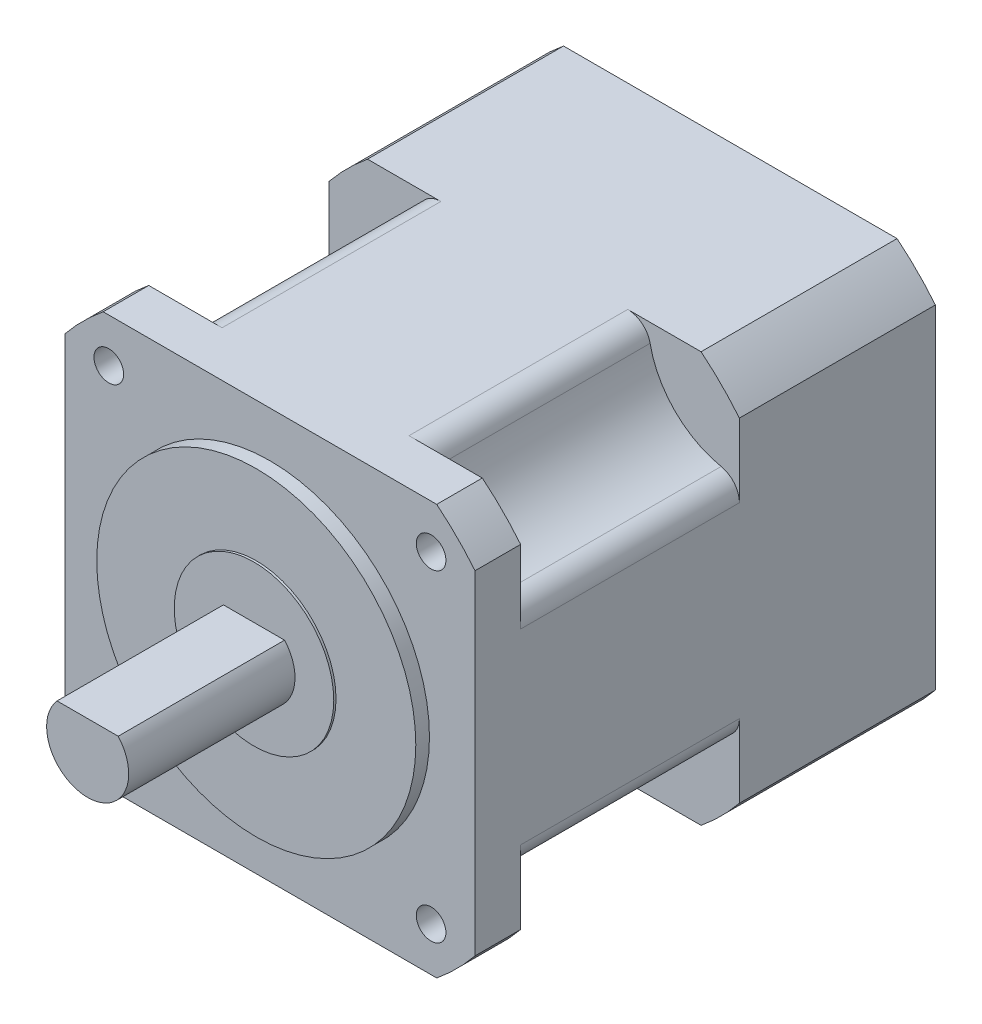
from build123d import *

# Parameters (mm, degrees)
SKETCH_1_W          = 90
SKETCH_1_H          = 90
EXTRUDE_1_DEPTH     = 10
SKETCH_2_R          = 35
EXTRUDE_2_DEPTH     = 3
SKETCH_3_R          = 17.5
EXTRUDE_3_DEPTH     = 0.5
EXTRUDE_4_DEPTH     = 36.5
CUT_EXTRUDE_1_REACH = 135.417
SKETCH_5_R          = 3.25
SKETCH_7_W          = 90
SKETCH_7_H          = 90
EXTRUDE_5_DEPTH     = 91
SKETCH_8_R          = 20
CUT_EXTRUDE_2_DEPTH = 48
FILLET_1_R          = 5
SKETCH_6_OUTSIDE_W  = 129.99
SKETCH_6_OUTSIDE_H  = 129.99
SKETCH_6_OUTSIDE_R  = 58
CUT_EXTRUDE_3_DEPTH = 163.483845351


with BuildPart() as part:
    # 草图1 → 拉伸1 (new body)
    with BuildSketch(Plane.XY):
        with Locations((45, 45)):
            Rectangle(SKETCH_1_W, SKETCH_1_H)
    extrude(amount=EXTRUDE_1_DEPTH)

    # 草图2 → 拉伸2 (add)
    with BuildSketch(Plane.XY.offset(10)):
        with Locations(Location((45, 45, 0), (0, 0, 180))):
            Circle(SKETCH_2_R)
    extrude(amount=EXTRUDE_2_DEPTH)

    # 草图3 → 拉伸3 (add)
    with BuildSketch(Plane.XY.offset(13)):
        with Locations((45, 45)):
            Circle(SKETCH_3_R)
    extrude(amount=EXTRUDE_3_DEPTH)

    # 草图4 → 拉伸4 (add)
    with BuildSketch(Plane.XY.offset(13.5)):
        with BuildLine():
            Line((38.291796068, 51), (51.708203932, 51))
            ThreePointArc((51.708203932, 51), (45, 36), (38.291796068, 51))
        make_face()
    extrude(amount=EXTRUDE_4_DEPTH)

    # 草图5 → 切除-拉伸1 (cut, up to next)
    with BuildSketch(Plane.XY.offset(10), mode=Mode.PRIVATE) as cut_extrude_1_sk1:
        with Locations((9.644660941, 80.355339059)):
            Circle(SKETCH_5_R)
    cut_extrude_1_tool1 = extrude(cut_extrude_1_sk1.sketch, amount=-CUT_EXTRUDE_1_REACH, mode=Mode.PRIVATE) & part.part
    # 草图5 → 切除-拉伸1 (cut, up to next)
    with BuildSketch(Plane.XY.offset(10), mode=Mode.PRIVATE) as cut_extrude_1_sk2:
        with Locations(Location((80.355339059, 80.355339059, 0), (0, 0, 180))):
            Circle(SKETCH_5_R)
    cut_extrude_1_tool2 = extrude(cut_extrude_1_sk2.sketch, amount=-CUT_EXTRUDE_1_REACH, mode=Mode.PRIVATE) & part.part
    # 草图5 → 切除-拉伸1 (cut, up to next)
    with BuildSketch(Plane.XY.offset(10), mode=Mode.PRIVATE) as cut_extrude_1_sk3:
        with Locations((80.355339059, 9.644660941)):
            Circle(SKETCH_5_R)
    cut_extrude_1_tool3 = extrude(cut_extrude_1_sk3.sketch, amount=-CUT_EXTRUDE_1_REACH, mode=Mode.PRIVATE) & part.part
    # 草图5 → 切除-拉伸1 (cut, up to next)
    with BuildSketch(Plane.XY.offset(10), mode=Mode.PRIVATE) as cut_extrude_1_sk4:
        with Locations(Location((9.644660941, 9.644660941, 0), (0, 0, 180))):
            Circle(SKETCH_5_R)
    cut_extrude_1_tool4 = extrude(cut_extrude_1_sk4.sketch, amount=-CUT_EXTRUDE_1_REACH, mode=Mode.PRIVATE) & part.part
    add(cut_extrude_1_tool1.solids().sort_by_distance((9.644661, 80.355339, 10))[0], mode=Mode.SUBTRACT)
    add(cut_extrude_1_tool2.solids().sort_by_distance((80.355339, 80.355339, 10))[0], mode=Mode.SUBTRACT)
    add(cut_extrude_1_tool3.solids().sort_by_distance((80.355339, 9.644661, 10))[0], mode=Mode.SUBTRACT)
    add(cut_extrude_1_tool4.solids().sort_by_distance((9.644661, 9.644661, 10))[0], mode=Mode.SUBTRACT)

    # 草图7 → 拉伸5 (add)
    with BuildSketch(Plane(origin=(0, 0, 0), x_dir=(-1, 0, 0), z_dir=(0, 0, -1))):
        with Locations((-45, 45)):
            Rectangle(SKETCH_7_W, SKETCH_7_H)
    extrude(amount=EXTRUDE_5_DEPTH)

    # 草图8 → 切除-拉伸2 (cut)
    with BuildSketch(Plane.XY):
        with Locations((90, 90)):
            Circle(SKETCH_8_R)
        with Locations((90, 0)):
            Circle(SKETCH_8_R)
        Circle(SKETCH_8_R)
        with Locations((0, 90)):
            Circle(SKETCH_8_R)
    extrude(amount=-CUT_EXTRUDE_2_DEPTH, mode=Mode.SUBTRACT)

    # 圆角1
    fillet_1_edges = [part.edges().sort_by_distance(p)[0] for p in [
        (70, 90, -24),
        (90, 70, -24),
        (70, 0, -24),
        (90, 20, -24),
        (20, 0, -24),
        (0, 20, -24),
        (20, 90, -24),
        (0, 70, -24),
    ]]
    fillet(fillet_1_edges, radius=FILLET_1_R)

    # 草图6 outside → 切除-拉伸3 (cut, through all)
    with BuildSketch(Plane.XY.offset(10)):
        with Locations((45, 45)):
            Rectangle(SKETCH_6_OUTSIDE_W, SKETCH_6_OUTSIDE_H)
        with Locations((45, 45)):
            Circle(SKETCH_6_OUTSIDE_R, mode=Mode.SUBTRACT)
    extrude(amount=-CUT_EXTRUDE_3_DEPTH, mode=Mode.SUBTRACT)


solid = part.part
